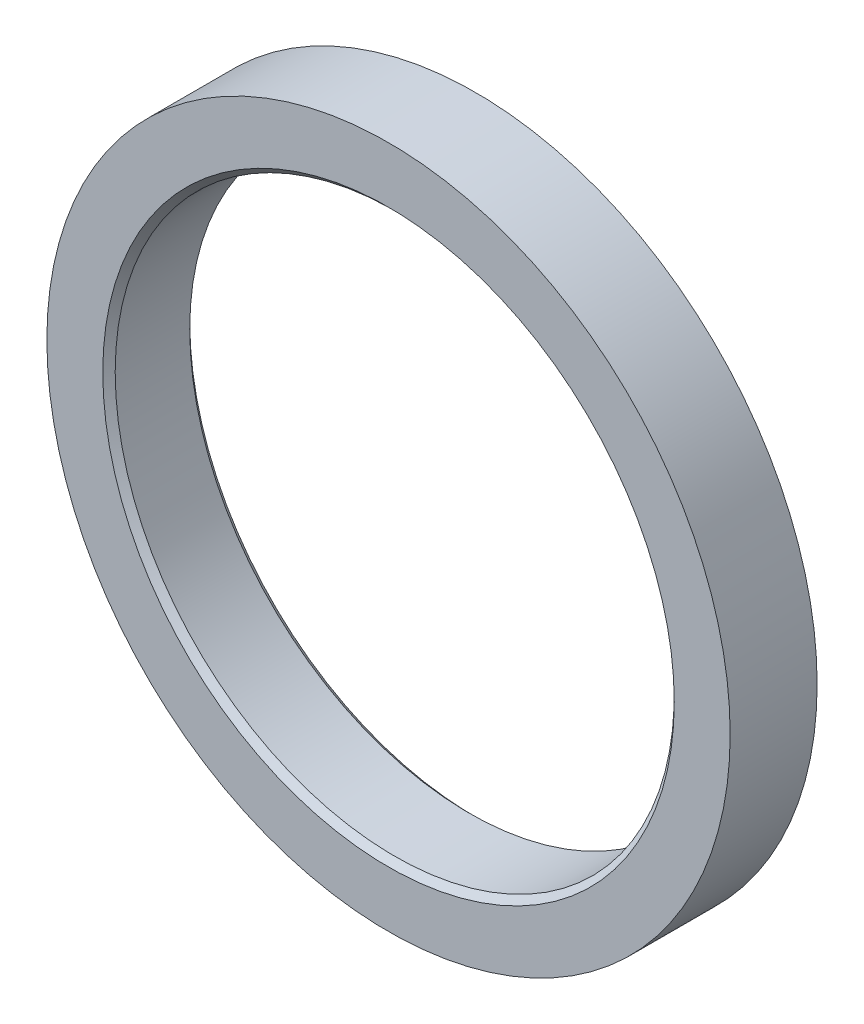
from build123d import *


with BuildPart() as part:
    # Sketch1 → Revolve1 (revolve)
    with BuildSketch(Plane.XZ.offset(-40.2756484), mode=Mode.PRIVATE) as revolve1_sk:
        Polygon((475.77422742, -188.192981355), (476.27422742, -188.692981355), (480.77422742, -188.692981355), (480.77422742, -181.692981355), (476.27422742, -181.692981355), (475.77422742, -182.192981355), align=None)
    revolve(revolve1_sk.sketch.rotate(Axis((453.27422742, 40.2756484, -181.692981355), (0, 0, -1)), 180), axis=Axis((453.27422742, 40.2756484, -181.692981355), (0, 0, -1)))


solid = part.part
